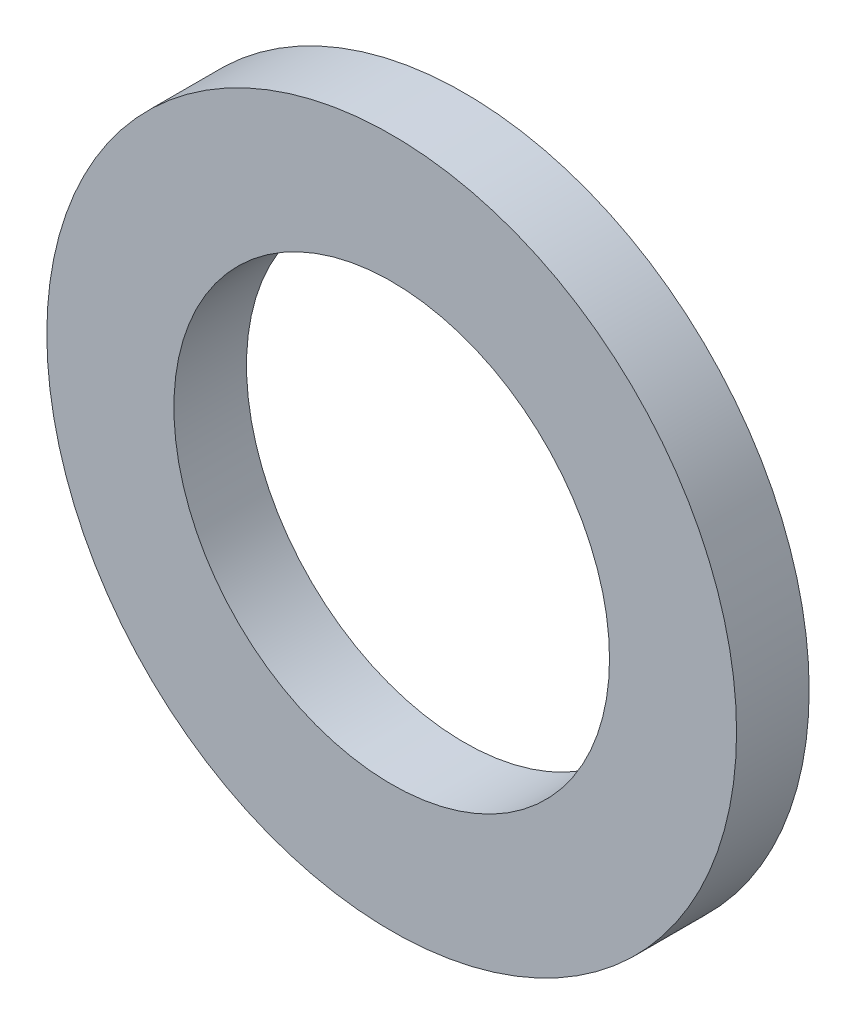
from build123d import *

# Parameters (mm, degrees)
SKETCH1_R           = 38
SKETCH1_R_2         = 24
BOSS_EXTRUDE1_DEPTH = 8


with BuildPart() as part:
    # Sketch1 → Boss-Extrude1 (new body)
    with BuildSketch(Plane.XY):
        Circle(SKETCH1_R)
        Circle(SKETCH1_R_2, mode=Mode.SUBTRACT)
    extrude(amount=BOSS_EXTRUDE1_DEPTH)


solid = part.part
